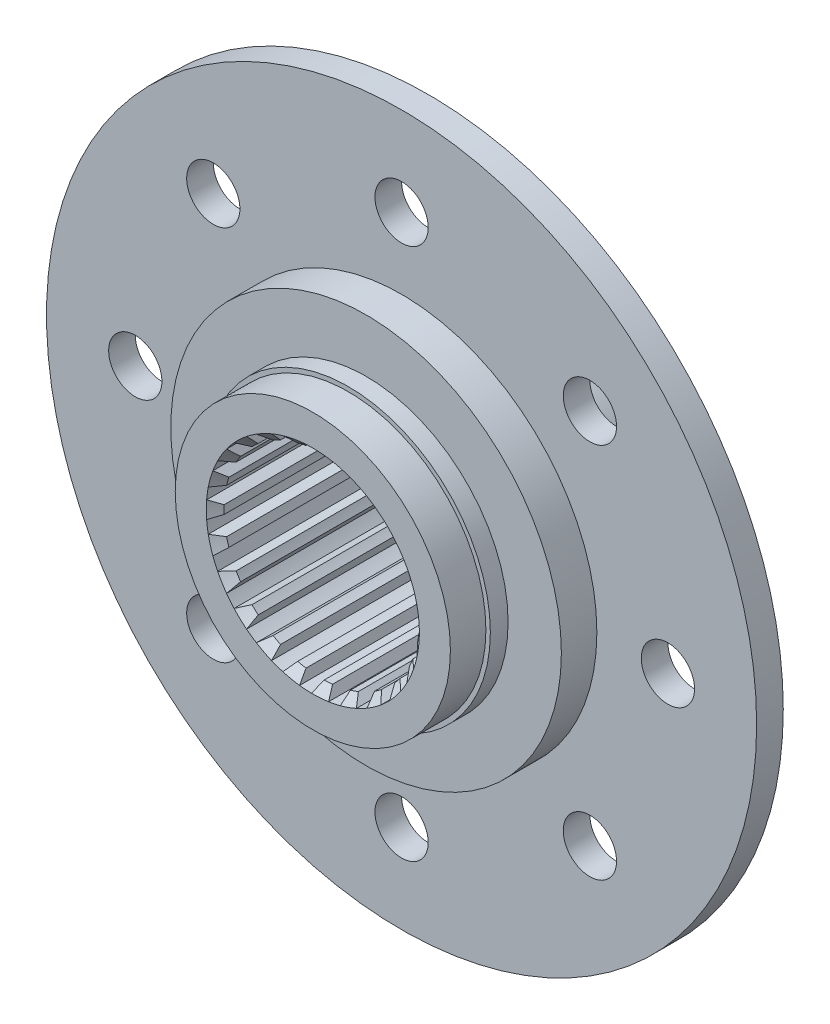
from build123d import *

# Parameters (mm, degrees)
SKETCH1_R           = 40
BOSS_EXTRUDE1_DEPTH = 3
SKETCH2_R           = 18
BOSS_EXTRUDE2_DEPTH = 1
SKETCH3_R           = 16
BOSS_EXTRUDE3_DEPTH = 3
SKETCH4_R           = 15.5
BOSS_EXTRUDE4_DEPTH = 9
SKETCH5_R           = 22
BOSS_EXTRUDE5_DEPTH = 4
BOSS_EXTRUDE6_START = 2
SKETCH6_R           = 16
BOSS_EXTRUDE6_DEPTH = 2
BOSS_EXTRUDE7_START = 4
SKETCH7_R           = 15.5
BOSS_EXTRUDE7_DEPTH = 4
SKETCH8_R           = 3
CUT_EXTRUDE1_DEPTH  = 12
SKETCH10_R          = 12
CUT_EXTRUDE2_DEPTH  = 33
BOSS_EXTRUDE8_DEPTH = 26


with BuildPart() as part:
    # Sketch1 → Boss-Extrude1 (new body)
    with BuildSketch(Plane.XY):
        Circle(SKETCH1_R)
    extrude(amount=BOSS_EXTRUDE1_DEPTH)

    # Sketch2 → Boss-Extrude2 (add)
    with BuildSketch(Plane(origin=(0, 0, 0), x_dir=(-1, 0, 0), z_dir=(0, 0, -1))):
        Circle(SKETCH2_R)
    extrude(amount=BOSS_EXTRUDE2_DEPTH)

    # Sketch3 → Boss-Extrude3 (add)
    with BuildSketch(Plane(origin=(0, 0, -1), x_dir=(-1, 0, 0), z_dir=(0, 0, -1))):
        Circle(SKETCH3_R)
    extrude(amount=BOSS_EXTRUDE3_DEPTH)

    # Sketch4 → Boss-Extrude4 (add)
    with BuildSketch(Plane(origin=(0, 0, -4), x_dir=(-1, 0, 0), z_dir=(0, 0, -1))):
        Circle(SKETCH4_R)
    extrude(amount=BOSS_EXTRUDE4_DEPTH)

    # Sketch5 → Boss-Extrude5 (add)
    with BuildSketch(Plane.XY.offset(3)):
        Circle(SKETCH5_R)
    extrude(amount=BOSS_EXTRUDE5_DEPTH)

    # Sketch6 → Boss-Extrude6 (add)
    with BuildSketch(Plane.XY.offset(7).offset(BOSS_EXTRUDE6_START)):
        with Locations(Location((0, 0, 0), (0, 0, 180))):
            Circle(SKETCH6_R)
    extrude(amount=-BOSS_EXTRUDE6_DEPTH)

    # Sketch7 → Boss-Extrude7 (add)
    with BuildSketch(Plane.XY.offset(9).offset(BOSS_EXTRUDE7_START)):
        with Locations(Location((0, 0, 0), (0, 0, 180))):
            Circle(SKETCH7_R)
    extrude(amount=-BOSS_EXTRUDE7_DEPTH)

    # Sketch8 → Cut-Extrude1 (cut)
    with BuildSketch(Plane(origin=(0, 0, 0), x_dir=(-1, 0, 0), z_dir=(0, 0, -1))):
        with Locations((0, 30)):
            Circle(SKETCH8_R)
        with Locations((21.213203436, 21.213203436)):
            Circle(SKETCH8_R)
        with Locations((30, 0)):
            Circle(SKETCH8_R)
        with Locations((21.213203436, -21.213203436)):
            Circle(SKETCH8_R)
        with Locations((0, -30)):
            Circle(SKETCH8_R)
        with Locations((-21.213203436, -21.213203436)):
            Circle(SKETCH8_R)
        with Locations((-30, 0)):
            Circle(SKETCH8_R)
        with Locations((-21.213203436, 21.213203436)):
            Circle(SKETCH8_R)
    extrude(amount=-CUT_EXTRUDE1_DEPTH, mode=Mode.SUBTRACT)

    # Sketch10 → Cut-Extrude2 (cut)
    with BuildSketch(Plane(origin=(0, 0, -13), x_dir=(-1, 0, 0), z_dir=(0, 0, -1))):
        Circle(SKETCH10_R)
    extrude(amount=-CUT_EXTRUDE2_DEPTH, mode=Mode.SUBTRACT)

    # Sketch11 → Boss-Extrude8 (add)
    with BuildSketch(Plane(origin=(0, 0, -13), x_dir=(-1, 0, 0), z_dir=(0, 0, -1))):
        with BuildLine():
            Line((-11.718692126, 2.583070821), (-10.822254184, 1.969470585))
            ThreePointArc((-10.822254184, 1.969470585), (-10.897545406, 1.49783314), (-10.952292446, 1.023371962))
            Line((-10.952292446, 1.023371962), (-11.9810354, 0.67438175))
            ThreePointArc((-11.9810354, 0.67438175), (-11.888231352, 1.633999789), (-11.718692126, 2.583070821))
        make_face()
        with BuildLine():
            Line((-10.587227066, 5.648948846), (-9.889578837, 4.816246509))
            ThreePointArc((-9.889578837, 4.816246509), (-10.089324317, 4.382411988), (-10.270049282, 3.940315692))
            Line((-10.270049282, 3.940315692), (-11.354800088, 3.881818511))
            ThreePointArc((-11.354800088, 3.881818511), (-11.006535618, 4.780813078), (-10.587227066, 5.648948846))
        make_face()
        with BuildLine():
            Line((-8.670555808, 8.295870177), (-8.223438669, 7.305823462))
            ThreePointArc((-8.223438669, 7.305823462), (-8.532824198, 6.941967388), (-8.826123544, 6.565024234))
            Line((-8.826123544, 6.565024234), (-9.886431199, 6.801358552))
            ThreePointArc((-9.886431199, 6.801358552), (-9.308535488, 7.573055332), (-8.670555808, 8.295870177))
        make_face()
        with BuildLine():
            Line((-6.110829091, 10.327524768), (-5.947403675, 9.25356091))
            ThreePointArc((-5.947403675, 9.25356091), (-6.343483543, 8.986668823), (-6.7276046, 8.70283496))
            Line((-6.7276046, 8.70283496), (-7.684830935, 9.216472943))
            ThreePointArc((-7.684830935, 9.216472943), (-6.920163865, 9.803638716), (-6.110829091, 10.327524768))
        make_face()
        with BuildLine():
            Line((-3.097890135, 11.593234092), (-3.230276959, 10.515004078))
            ThreePointArc((-3.230276959, 10.515004078), (-3.683675734, 10.364870143), (-4.13013, 10.195196231))
            Line((-4.13013, 10.195196231), (-4.913281916, 10.948043698))
            ThreePointArc((-4.913281916, 10.948043698), (-4.018555346, 11.307131065), (-3.097890135, 11.593234092))
        make_face()
        with BuildLine():
            Line((0.14480516, 11.999126279), (-0.273575377, 10.996597497))
            ThreePointArc((-0.273575377, 10.996597497), (-0.750666547, 10.974356461), (-1.226342551, 10.931426437))
            Line((-1.226342551, 10.931426437), (-1.777337254, 11.867648136))
            ThreePointArc((-1.777337254, 11.867648136), (-0.81890896, 11.97202523), (0.14480516, 11.999126279))
        make_face()
        with BuildLine():
            Line((3.376760919, 11.515098163), (2.703416038, 10.662623585))
            ThreePointArc((2.703416038, 10.662623585), (2.238016144, 10.769924965), (1.768397114, 10.856922752))
            Line((1.768397114, 10.856922752), (1.490424381, 11.907083403))
            ThreePointArc((1.490424381, 11.907083403), (2.441472157, 11.749009052), (3.376760919, 11.515098163))
        make_face()
        with BuildLine():
            Line((6.358277768, 10.177047894), (5.479907453, 9.537851661))
            ThreePointArc((5.479907453, 9.537851661), (5.060715415, 9.766737402), (4.631982855, 9.977210774))
            Line((4.631982855, 9.977210774), (4.647648058, 11.063424765))
            ThreePointArc((4.647648058, 11.063424765), (5.520780453, 10.654622621), (6.358277768, 10.177047894))
        make_face()
        with BuildLine():
            Line((8.868230242, 8.084212539), (7.849979202, 7.705700911))
            ThreePointArc((7.849979202, 7.705700911), (7.508084575, 8.039195607), (7.152035618, 8.357534715))
            Line((7.152035618, 8.357534715), (7.46017694, 9.399242524))
            ThreePointArc((7.46017694, 9.399242524), (8.190637719, 8.770031571), (8.868230242, 8.084212539))
        make_face()
        with BuildLine():
            Line((10.720466648, 5.391808123), (9.637853904, 5.302053576))
            ThreePointArc((9.637853904, 5.302053576), (9.39861345, 5.71542345), (9.141654617, 6.11801854))
            Line((9.141654617, 6.11801854), (9.719418626, 7.037961464))
            ThreePointArc((9.719418626, 7.037961464), (10.253032855, 6.2350074), (10.720466648, 5.391808123))
        make_face()
        with BuildLine():
            Line((11.777615087, 2.299517965), (10.710933072, 2.505177183))
            ThreePointArc((10.710933072, 2.505177183), (10.592090161, 2.967764483), (10.453278914, 3.424756918))
            Line((10.453278914, 3.424756918), (11.257815497, 4.154706998))
            ThreePointArc((11.257815497, 4.154706998), (11.555007448, 3.237561254), (11.777615087, 2.299517965))
        make_face()
        with BuildLine():
            Line((11.961271693, -0.963316921), (10.989631334, -0.477496742))
            ThreePointArc((10.989631334, -0.477496742), (11, 0), (10.989631334, 0.477496742))
            Line((10.989631334, 0.477496742), (11.961271693, 0.963316921))
            ThreePointArc((11.961271693, 0.963316921), (12, 0), (11.961271693, -0.963316921))
        make_face()
        with BuildLine():
            Line((11.257815497, -4.154706998), (10.453278914, -3.424756918))
            ThreePointArc((10.453278914, -3.424756918), (10.592090161, -2.967764483), (10.710933072, -2.505177183))
            Line((10.710933072, -2.505177183), (11.777615087, -2.299517965))
            ThreePointArc((11.777615087, -2.299517965), (11.555007448, -3.237561254), (11.257815497, -4.154706998))
        make_face()
        with BuildLine():
            Line((9.719418626, -7.037961464), (9.141654617, -6.11801854))
            ThreePointArc((9.141654617, -6.11801854), (9.39861345, -5.71542345), (9.637853904, -5.302053576))
            Line((9.637853904, -5.302053576), (10.720466648, -5.391808123))
            ThreePointArc((10.720466648, -5.391808123), (10.253032855, -6.2350074), (9.719418626, -7.037961464))
        make_face()
        with BuildLine():
            Line((7.46017694, -9.399242524), (7.152035618, -8.357534715))
            ThreePointArc((7.152035618, -8.357534715), (7.508084575, -8.039195607), (7.849979202, -7.705700911))
            Line((7.849979202, -7.705700911), (8.868230242, -8.084212539))
            ThreePointArc((8.868230242, -8.084212539), (8.190637719, -8.770031571), (7.46017694, -9.399242524))
        make_face()
        with BuildLine():
            Line((4.647648058, -11.063424765), (4.631982855, -9.977210774))
            ThreePointArc((4.631982855, -9.977210774), (5.060715415, -9.766737402), (5.479907453, -9.537851661))
            Line((5.479907453, -9.537851661), (6.358277768, -10.177047894))
            ThreePointArc((6.358277768, -10.177047894), (5.520780453, -10.654622621), (4.647648058, -11.063424765))
        make_face()
        with BuildLine():
            Line((1.490424381, -11.907083403), (1.768397114, -10.856922752))
            ThreePointArc((1.768397114, -10.856922752), (2.238016144, -10.769924965), (2.703416038, -10.662623585))
            Line((2.703416038, -10.662623585), (3.376760919, -11.515098163))
            ThreePointArc((3.376760919, -11.515098163), (2.441472157, -11.749009052), (1.490424381, -11.907083403))
        make_face()
        with BuildLine():
            Line((-1.777337254, -11.867648136), (-1.226342551, -10.931426437))
            ThreePointArc((-1.226342551, -10.931426437), (-0.750666547, -10.974356461), (-0.273575377, -10.996597497))
            Line((-0.273575377, -10.996597497), (0.14480516, -11.999126279))
            ThreePointArc((0.14480516, -11.999126279), (-0.81890896, -11.97202523), (-1.777337254, -11.867648136))
        make_face()
        with BuildLine():
            Line((-4.913281916, -10.948043698), (-4.13013, -10.195196231))
            ThreePointArc((-4.13013, -10.195196231), (-3.683675734, -10.364870143), (-3.230276959, -10.515004078))
            Line((-3.230276959, -10.515004078), (-3.097890135, -11.593234092))
            ThreePointArc((-3.097890135, -11.593234092), (-4.018555346, -11.307131065), (-4.913281916, -10.948043698))
        make_face()
        with BuildLine():
            Line((-7.684830935, -9.216472943), (-6.7276046, -8.70283496))
            ThreePointArc((-6.7276046, -8.70283496), (-6.343483543, -8.986668823), (-5.947403675, -9.25356091))
            Line((-5.947403675, -9.25356091), (-6.110829091, -10.327524768))
            ThreePointArc((-6.110829091, -10.327524768), (-6.920163865, -9.803638716), (-7.684830935, -9.216472943))
        make_face()
        with BuildLine():
            Line((-9.886431199, -6.801358552), (-8.826123544, -6.565024234))
            ThreePointArc((-8.826123544, -6.565024234), (-8.532824198, -6.941967388), (-8.223438669, -7.305823462))
            Line((-8.223438669, -7.305823462), (-8.670555808, -8.295870177))
            ThreePointArc((-8.670555808, -8.295870177), (-9.308535488, -7.573055332), (-9.886431199, -6.801358552))
        make_face()
        with BuildLine():
            Line((-11.354800088, -3.881818511), (-10.270049282, -3.940315692))
            ThreePointArc((-10.270049282, -3.940315692), (-10.089324317, -4.382411988), (-9.889578837, -4.816246509))
            Line((-9.889578837, -4.816246509), (-10.587227066, -5.648948846))
            ThreePointArc((-10.587227066, -5.648948846), (-11.006535618, -4.780813078), (-11.354800088, -3.881818511))
        make_face()
        with BuildLine():
            Line((-11.9810354, -0.67438175), (-10.952292446, -1.023371962))
            ThreePointArc((-10.952292446, -1.023371962), (-10.897545406, -1.49783314), (-10.822254184, -1.969470585))
            Line((-10.822254184, -1.969470585), (-11.718692126, -2.583070821))
            ThreePointArc((-11.718692126, -2.583070821), (-11.888231352, -1.633999789), (-11.9810354, -0.67438175))
        make_face()
    extrude(amount=-BOSS_EXTRUDE8_DEPTH)

    # Sketch12 → Cut-Revolve1 (revolve, cut)
    with BuildSketch(Plane(origin=(0, 0, 0), x_dir=(1, 0, 0), z_dir=(0, 1, 0)), mode=Mode.PRIVATE) as cut_revolve1_sk:
        Polygon((0, 13), (-12, 13), (-10, 11), (-8.510506148, 11), (0, 11), align=None)
        Polygon((0, -11), (0, -13), (-12, -13), (-10, -11), (-8.510506148, -11), align=None)
    revolve(cut_revolve1_sk.sketch.rotate(Axis((0, 0, -11), (0, 0, -1)), 180), axis=Axis((0, 0, -11), (0, 0, -1)), mode=Mode.SUBTRACT)


solid = part.part
